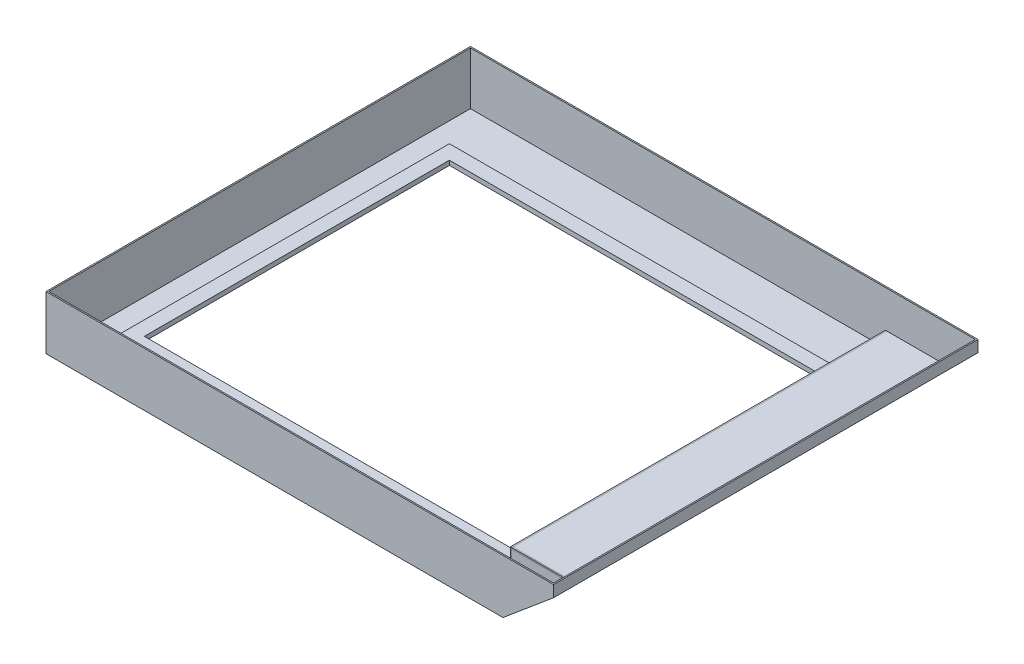
SolidWorks part; units mm, degrees
ref_plane "前视基准面" through (0, 0, 0) normal (0, 0, 1) x (1, 0, 0)
ref_plane "上视基准面" through (0, 0, 0) normal (0, 1, 0) x (1, 0, 0)
ref_plane "右视基准面" through (0, 0, 0) normal (1, 0, 0) x (0, 0, -1)
sketch "草图2" plane through (0, 0, 0) normal (0, 0, 1) x (1, 0, 0)
  line L0 (0, 0) -> (0, 83)
  line L1 (0, 83) -> (784, 83)
  line L3 (784, 67) -> (704.1525, 0)
  line L4 (704.1525, 0) -> (0, 0)
  line L5 (784, 83) -> (784, 67)
  dimension "D1" = 67
  dimension "D2" = 140
  dimension "D3" = 784
  dimension "D4" = 83
extrude "凸台-拉伸1" add sketch "草图2" along normal blind 654
sketch "草图8" plane through (0, 0, 654) normal (0, 0, 1) x (1, 0, 0)
  line L0 (784, 67) -> (784, 83) construction
  line L1 (782, 134.1526) -> (892.0044, 134.1526)
  line L2 (782, 134.1526) -> (782, 0)
  line L3 (782, 0) -> (892.0044, 0)
  line L4 (892.0044, 134.1526) -> (892.0044, 0)
  dimension "D1" = 2
extrude "切除-拉伸2" cut sketch "草图8" against normal blind 799
shell "抽壳1" thickness 2
sketch "草图3" plane through (290.9389, -346.7274, 0) normal (0.6428, -0.766, 0) x (0.766, 0.6428, 0)
  line L0 (539.4121, 327) -> (815.6504, 327) construction
  line L1 (539.4121, 654) -> (539.4121, 0) construction
  line L2 (590.2235, 654) -> (590.2235, -41.4419) construction
  line L3 (539.4121, 654) -> (641.0348, 654) construction
  line L5 (552.7235, 614) -> (627.7235, 614)
  line L6 (552.7235, 614) -> (552.7235, 40)
  line L7 (552.7235, 40) -> (627.7235, 40)
  line L8 (627.7235, 614) -> (627.7235, 40)
  dimension "D1" = 287
  dimension "D2" = 574
  dimension "D3" = 37.5
  dimension "D4" = 75
extrude "切除-拉伸1" cut sketch "草图3" against normal blind 654
sketch "草图5" plane through (0, 2, 0) normal (0, 1, 0) x (1, 0, 0)
  line L0 (2, -327) -> (979.0478, -327) construction
  line L1 (677.4246, -38) -> (679.4246, -38)
  line L2 (677.4246, -38) -> (677.4246, -616)
  line L3 (677.4246, -616) -> (679.4246, -616)
  line L4 (679.4246, -38) -> (679.4246, -616)
  line L5 (2, -652) -> (2, -2) construction
  line L6 (703.4246, -652) -> (703.4246, -2) construction
  dimension "D1" = 2
  dimension "D2" = 24
  dimension "D3" = 578
  dimension "D4" = 289
extrude "凸台-拉伸2" add sketch "草图5" along normal blind 60
ref_plane "基准面1" through (0, 0, 327) normal (0, 0, 1) x (1, 0, 0)
sketch "草图6" plane through (0, 0, 327) normal (0, 0, 1) x (1, 0, 0)
  line L0 (679.4246, 62) -> (774.9298, 62)
  line L1 (703.4246, 2) -> (780, 66.2544) construction
  line L2 (774.9298, 62) -> (772.5463, 60)
  line L16 (681.4246, 62) -> (681.4246, 2)
  line L17 (681.4246, 60) -> (681.4246, 4)
  line L21 (681.4246, 60) -> (772.5463, 60)
  line L22 (702.139, 3.5321) -> (778.7144, 67.7865)
  line L23 (702.6966, 4) -> (746.2504, 40.546)
  line L24 (679.4246, 62) -> (679.4246, 2)
  line L25 (679.4246, 2) -> (703.4246, 2)
  line L26 (703.4246, 2) -> (747.536, 39.0139)
  line L27 (747.536, 39.0139) -> (746.2504, 40.546)
  line L28 (681.4246, 4) -> (702.6966, 4)
  line L29 (679.4246, 60) -> (774.9298, 60) construction
  line L30 (770.5173, 58.2975) -> (771.8029, 56.7654) construction
  dimension "D2" = 2
  dimension "D5" = 30
  dimension "D1" = 2
  dimension "D3" = 2
  dimension "D4" = 2
extrude "凸台-拉伸3" add sketch "草图6" along normal blind 289 and the other way blind 289 separate body
sketch "草图9" plane through (0, 0, 616) normal (0, 0, 1) x (1, 0, 0)
  line L0 (679.4246, 62) -> (679.4246, 2)
  line L1 (679.4246, 2) -> (703.4246, 2)
  line L2 (703.4246, 2) -> (774.9298, 62)
  line L3 (774.9298, 62) -> (679.4246, 62)
extrude "凸台-拉伸5" add sketch "草图9" against normal blind 2 separate body
sketch "草图10" plane through (0, 0, 38) normal (0, 0, -1) x (-1, 0, 0)
  line L0 (-679.4246, 2) -> (-679.4246, 62)
  line L1 (-679.4246, 62) -> (-774.9298, 62)
  line L2 (-774.9298, 62) -> (-703.4246, 2)
  line L3 (-703.4246, 2) -> (-679.4246, 2)
extrude "凸台-拉伸6" add sketch "草图10" against normal blind 2 separate body
sketch "草图11" plane through (0, 0, 0) normal (0, -1, 0) x (1, 0, 0)
  line L0 (352.0763, 654) -> (352.0763, -40.1781) construction
  line L1 (0, 654) -> (704.1525, 654) construction
  line L2 (0, 327) -> (908.3489, 327) construction
  line L3 (0, 654) -> (0, 0) construction
  line L5 (59.5763, 562) -> (644.5763, 562)
  line L6 (59.5763, 562) -> (59.5763, 92)
  line L7 (59.5763, 92) -> (644.5763, 92)
  line L8 (644.5763, 562) -> (644.5763, 92)
  dimension "D1" = 470
  dimension "D2" = 235
  dimension "D3" = 292.5
  dimension "D4" = 585
extrude "切除-拉伸3" cut sketch "草图11" against normal blind 2
sketch "草图12" plane through (0, 2, 0) normal (0, 1, 0) x (1, 0, 0)
  line L20 (646.5763, -90) -> (57.5763, -90)
  line L21 (57.5763, -90) -> (57.5763, -564)
  line L22 (57.5763, -564) -> (646.5763, -564)
  line L23 (646.5763, -564) -> (646.5763, -90)
  line L24 (644.5763, -562) -> (644.5763, -92)
  line L25 (59.5763, -562) -> (644.5763, -562)
  line L26 (59.5763, -92) -> (59.5763, -562)
  line L27 (644.5763, -92) -> (59.5763, -92)
  line L28 (644.5763, -562) -> (644.5763, -92)
  line L29 (59.5763, -562) -> (644.5763, -562)
  line L30 (59.5763, -92) -> (59.5763, -562)
  line L31 (644.5763, -92) -> (59.5763, -92)
  dimension "D1" = 0
  dimension "D2" = 2
extrude "凸台-拉伸7" add sketch "草图12" along normal blind 5
sketch "草图15" plane through (0, 7, 0) normal (0, 1, 0) x (1, 0, 0)
  line L10 (666.5763, -584) -> (666.5763, -70)
  line L11 (666.5763, -70) -> (37.5763, -70)
  line L12 (37.5763, -70) -> (37.5763, -584)
  line L13 (37.5763, -584) -> (666.5763, -584)
  line L14 (59.5763, -562) -> (644.5763, -562)
  line L15 (644.5763, -562) -> (644.5763, -92)
  line L16 (59.5763, -92) -> (59.5763, -562)
  line L17 (644.5763, -92) -> (59.5763, -92)
  line L18 (59.5763, -562) -> (644.5763, -562)
  line L19 (644.5763, -562) -> (644.5763, -92)
  line L20 (59.5763, -92) -> (59.5763, -562)
  line L21 (644.5763, -92) -> (59.5763, -92)
  dimension "D1" = 0
  dimension "D2" = 22
extrude "凸台-拉伸8" add sketch "草图15" against normal blind 2
